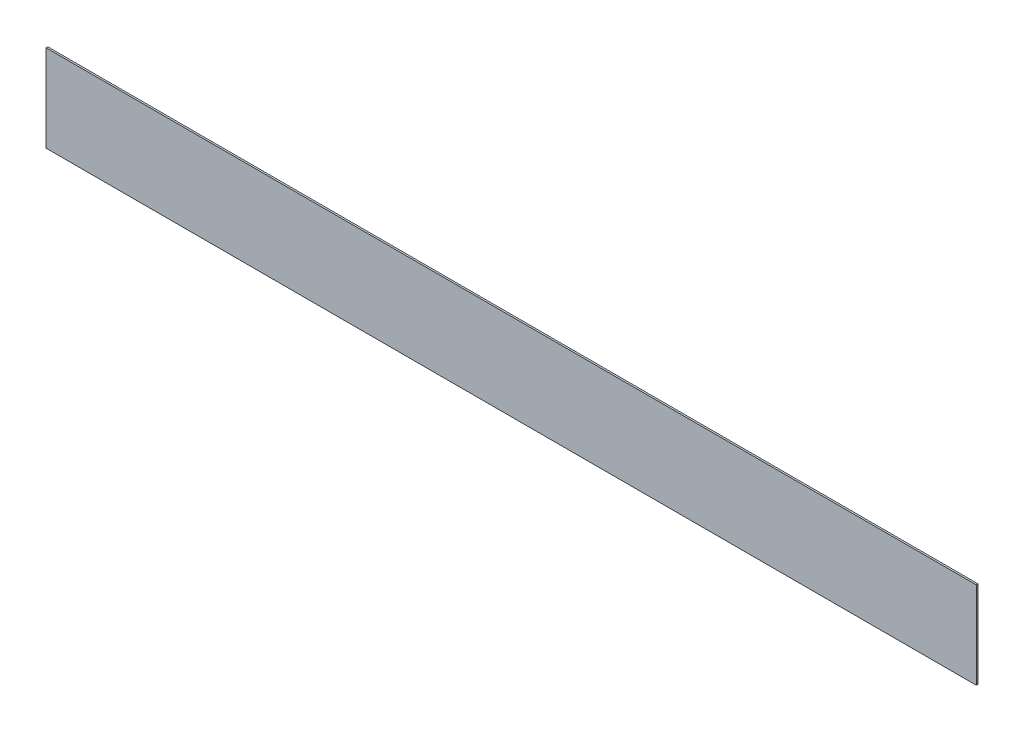
SolidWorks part; units mm, degrees
material "有机玻璃 (PMMA)"
ref_plane "前视" through (0, 0, 0) normal (0, 0, 1) x (1, 0, 0)
ref_plane "上视" through (0, 0, 0) normal (0, 1, 0) x (1, 0, 0)
ref_plane "右视" through (0, 0, 0) normal (1, 0, 0) x (0, 0, -1)
sketch "草图1" plane through (0, 0, 0) normal (0, 0, 1) x (1, 0, 0)
  line L1 (1070, -100) -> (-1070, -100)
  line L2 (1070, -100) -> (1070, 100)
  line L3 (1070, 100) -> (-1070, 100)
  line L4 (-1070, -100) -> (-1070, 100)
  line L5 (1070, -100) -> (-1070, 100) construction
  line L6 (1070, 100) -> (-1070, -100) construction
  point P0 (0, 0)
  dimension "D1" = 2140
  dimension "D2" = 200
extrude "凸台-拉伸1" add sketch "草图1" along normal blind 4
